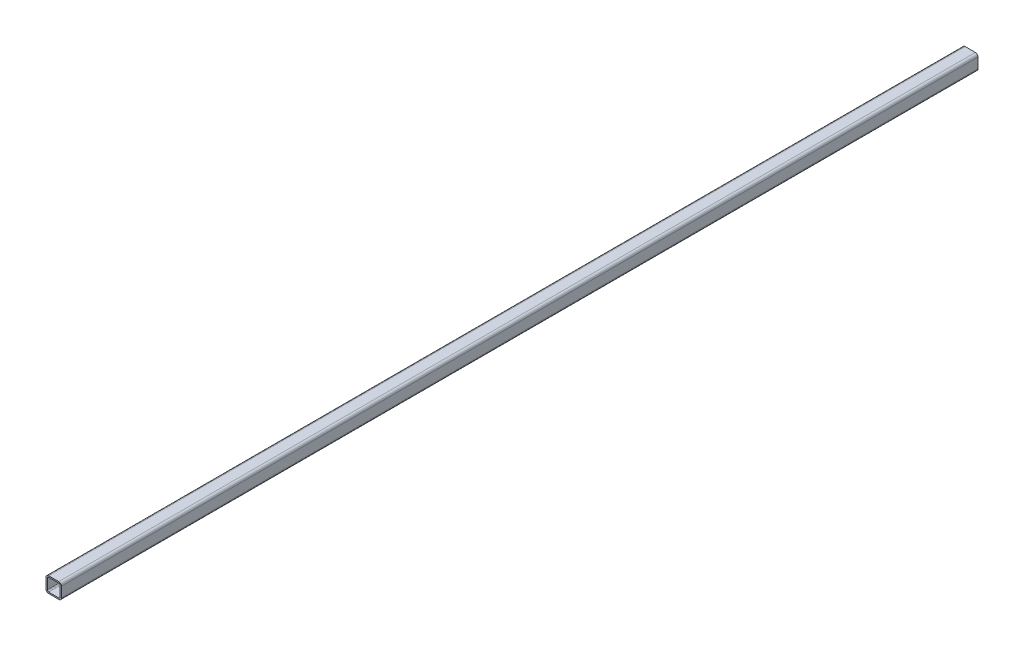
SolidWorks part; units mm, degrees
material "方管70×6/不锈钢304"
ref_plane "Front Plane" through (0, 0, 0) normal (0, 0, 1) x (1, 0, 0)
ref_plane "Top Plane" through (0, 0, 0) normal (0, 1, 0) x (1, 0, 0)
ref_plane "Right Plane" through (0, 0, 0) normal (1, 0, 0) x (0, 0, -1)
sketch "Sketch1" plane through (0, 0, 0) normal (0, 0, 1) x (1, 0, 0)
  line L1 (12, 0) -> (58, 0)
  line L2 (0, 12) -> (0, 58)
  line L3 (12, 70) -> (58, 70)
  line L4 (70, 12) -> (70, 58)
  line L5 (12, 6) -> (58, 6)
  line L6 (6, 12) -> (6, 58)
  line L7 (12, 64) -> (58, 64)
  line L8 (64, 12) -> (64, 58)
  arc A0 (12, 6) -> (6, 12) centre (12, 12) cw
  arc A1 (58, 6) -> (64, 12) centre (58, 12) ccw
  arc A2 (58, 64) -> (64, 58) centre (58, 58) cw
  arc A3 (6, 58) -> (12, 64) centre (12, 58) cw
  arc A4 (12, 0) -> (0, 12) centre (12, 12) cw
  arc A5 (58, 0) -> (70, 12) centre (58, 12) ccw
  arc A6 (58, 70) -> (70, 58) centre (58, 58) cw
  arc A7 (0, 58) -> (12, 70) centre (12, 58) cw
  point P19 (0, 0)
  point P22 (70, 0)
  point P27 (0, 70)
  dimension "D7" = 6
  dimension "D8" = 12
  dimension "D1" = 70
  dimension "D2" = 70
  dimension "D3" = 6
  dimension "D4" = 6
  dimension "D5" = 6
  dimension "D6" = 6
extrude "Boss-Extrude1" add sketch "Sketch1" along normal blind 4160
